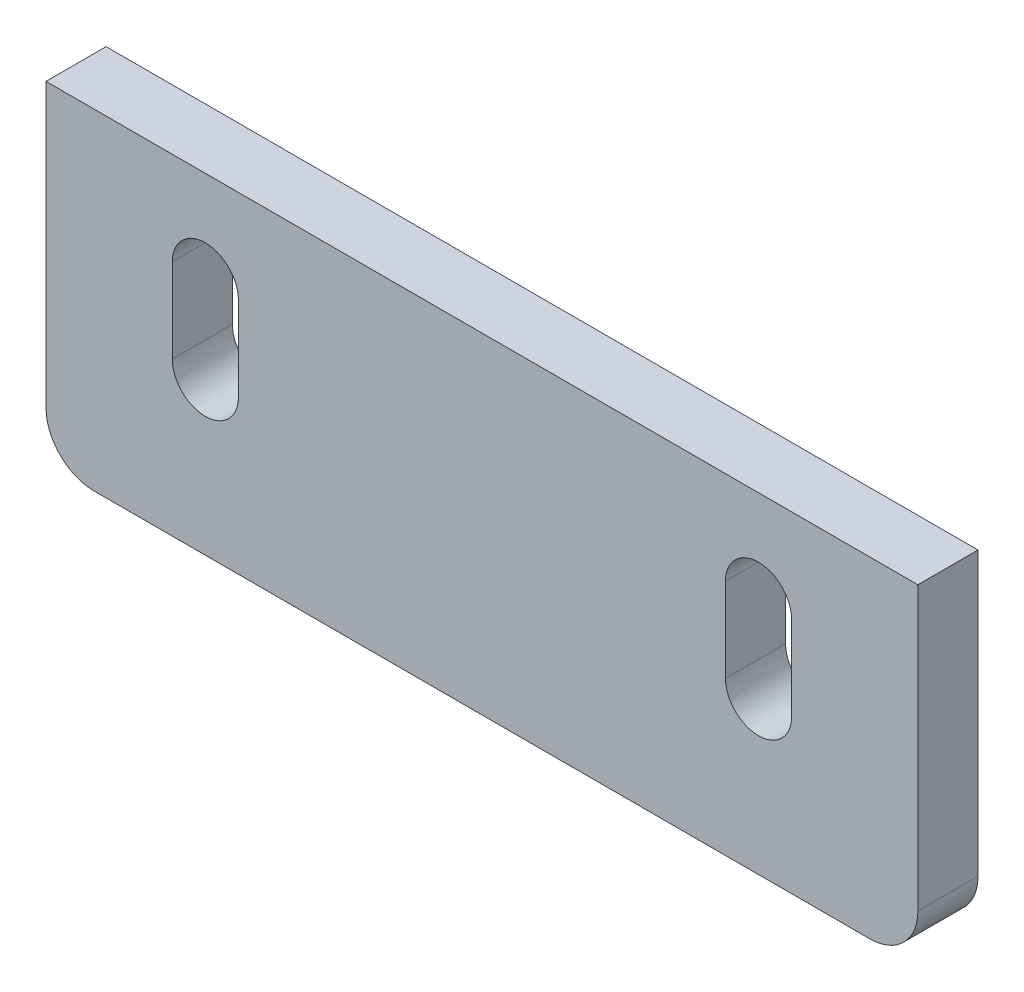
SolidWorks part; units mm, degrees
material "1023 碳钢板 (SS)"
ref_plane "前视基准面" through (0, 0, 0) normal (0, 0, 1) x (1, 0, 0)
ref_plane "上视基准面" through (0, 0, 0) normal (0, 1, 0) x (1, 0, 0)
ref_plane "右视基准面" through (0, 0, 0) normal (1, 0, 0) x (0, 0, -1)
sketch "草图1" plane through (0, 0, 0) normal (0, 0, 1) x (1, 0, 0)
  line L1 (72.5, 27.5) -> (-72.5, 27.5)
  line L2 (72.5, 27.5) -> (72.5, -27.5)
  line L3 (72.5, -27.5) -> (-72.5, -27.5)
  line L4 (-72.5, 27.5) -> (-72.5, -27.5)
  line L5 (72.5, 27.5) -> (-72.5, -27.5) construction
  line L6 (72.5, -27.5) -> (-72.5, 27.5) construction
  point P0 (0, 0)
  dimension "D1" = 145
  dimension "D2" = 55
extrude "凸台-拉伸1" add sketch "草图1" along normal blind 10
fillet "圆角1" radius 8 2 edges at (72.5, -27.5, 5) (-72.5, -27.5, 5)
sketch "草图2" plane through (0, 0, 10) normal (0, 0, 1) x (1, 0, 0)
  line L0 (46, 12) -> (46, -2) construction
  line L1 (51.5, 12) -> (51.5, -2)
  line L2 (40.5, 12) -> (40.5, -2)
  line L3 (-46, 12) -> (-46, -2) construction
  line L4 (-40.5, 12) -> (-40.5, -2)
  line L5 (-51.5, 12) -> (-51.5, -2)
  line L6 (72.5, 27.5) -> (-72.5, 27.5) construction
  line L7 (72.5, -19.5) -> (72.5, 27.5) construction
  arc A0 (51.5, 12) -> (40.5, 12) centre (46, 12) ccw
  arc A1 (40.5, -2) -> (51.5, -2) centre (46, -2) ccw
  arc A2 (-40.5, 12) -> (-51.5, 12) centre (-46, 12) ccw
  arc A3 (-51.5, -2) -> (-40.5, -2) centre (-46, -2) ccw
  point P2 (46, 5)
  point P7 (-46, 5)
  dimension "D1" = 5.5
  dimension "D4" = 26.5
  dimension "D2" = 14
  dimension "D3" = 92
  dimension "D5" = 15.5
extrude "切除-拉伸1" cut sketch "草图2" against normal blind 10
